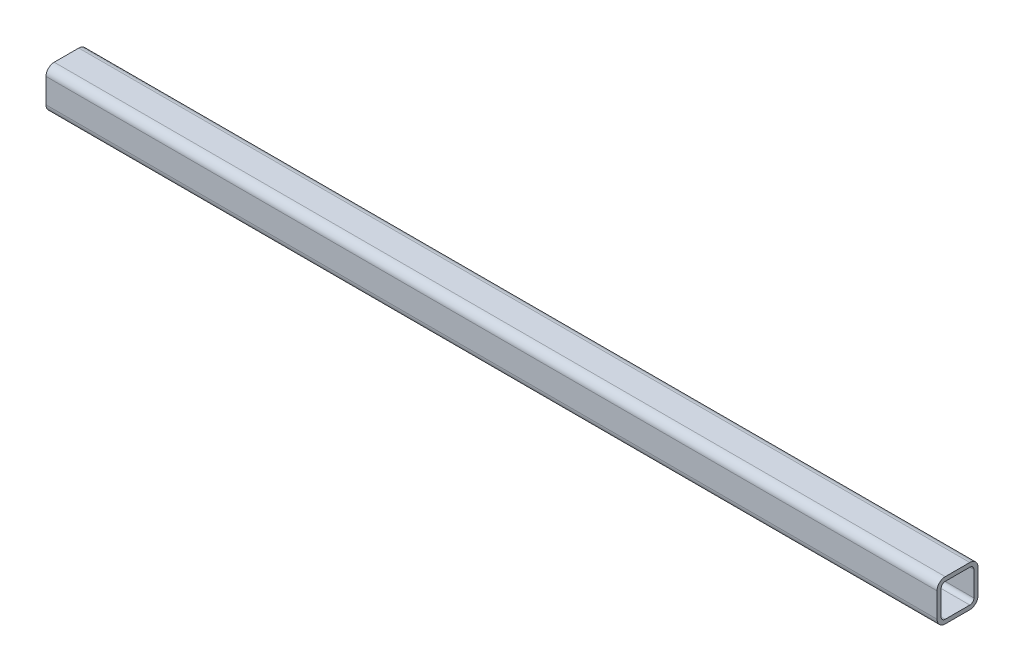
SolidWorks part; units mm, degrees
material "普通碳钢"
ref_plane "Front Plane" through (0, 0, 0) normal (0, 0, 1) x (1, 0, 0)
ref_plane "Top Plane" through (0, 0, 0) normal (0, 1, 0) x (1, 0, 0)
ref_plane "Right Plane" through (0, 0, 0) normal (1, 0, 0) x (0, 0, -1)
sketch "草图1" plane through (0, 0, 0) normal (0, 0, 1) x (1, 0, 0)
  line L0 (-1000, 0) -> (-130, 0)
  dimension "D1" = 870
  dimension "D2" = 1000
other "Square Tube 40 X 40 X 4(1)"
ref_plane "Plane1" through (-1000, 0, 0) normal (1, 0, 0) x (0, 1, 0)
sketch "Sketch1" plane through (-1000, 0, 0) normal (1, 0, 0) x (0, 1, 0)
  line L0 (-12, -16) -> (12, -16)
  line L1 (-16, -12) -> (-16, 12)
  line L2 (12, 16) -> (-12, 16)
  line L3 (16, 12) -> (16, -12)
  line L4 (-12, -20) -> (12, -20)
  line L5 (-20, -12) -> (-20, 12)
  line L6 (12, 20) -> (-12, 20)
  line L7 (20, 12) -> (20, -12)
  arc A0 (20, 12) -> (12, 20) centre (12, 12) ccw
  arc A1 (12, -20) -> (20, -12) centre (12, -12) ccw
  arc A2 (-20, -12) -> (-12, -20) centre (-12, -12) ccw
  arc A3 (-12, 20) -> (-20, 12) centre (-12, 12) ccw
  arc A4 (-12, 16) -> (-16, 12) centre (-12, 12) ccw
  arc A5 (16, 12) -> (12, 16) centre (12, 12) ccw
  arc A6 (12, -16) -> (16, -12) centre (12, -12) ccw
  arc A7 (-16, -12) -> (-12, -16) centre (-12, -12) ccw
  point P0 (-20, 0)
  point P1 (20, 0)
  point P2 (0, 20)
  point P3 (0, -20)
  point P4 (0, 0)
  point P5 (-20, -20)
  point P6 (20, -20)
  point P7 (20, 20)
  point P8 (-20, 20)
  point P33 (0, 0)
  dimension "D1" = 8
  dimension "Thickness" = 4
  dimension "V_leg" = 40
